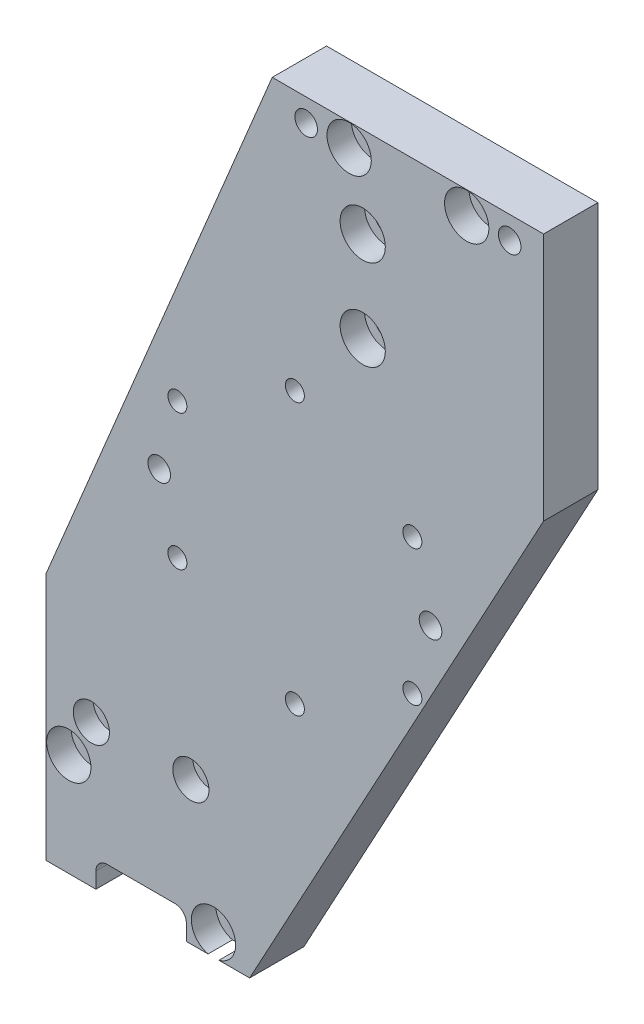
from build123d import *

# Parameters (mm, degrees)
SKETCH_1_W                   = 110
SKETCH_1_H                   = 175
EXTRUDE_1_DEPTH              = 6
CHAMFER_1_SIZE               = 50
CHAMFER_1_SIZE2              = 120
CHAMFER_2_SIZE               = 65
CHAMFER_2_SIZE2              = 120
HOLE_WIZARD_M5_1_D           = 5
HOLE_WIZARD_M5_1_2_D         = 4.2
F_5_0MM_1_D                  = 5
HOLE_WIZARD_M5_3_D           = 5.5
HOLE_WIZARD_M5_3_CBORE_D     = 9.8
HOLE_WIZARD_M5_3_CBORE_DEPTH = 5.4
HOLE_WIZARD_M5_4_D           = 5.5
HOLE_WIZARD_M5_4_CBORE_D     = 10
HOLE_WIZARD_M5_4_CBORE_DEPTH = 5.4
HOLE_WIZARD_M4_1_D           = 4.5
HOLE_WIZARD_M4_1_CBORE_D     = 8
HOLE_WIZARD_M4_1_CBORE_DEPTH = 4.4
HOLE_WIZARD_M5_6_D           = 5.5
HOLE_WIZARD_M5_6_CBORE_D     = 9.8
HOLE_WIZARD_M5_6_CBORE_DEPTH = 5.4
SKETCH_16_W                  = 20
SKETCH_16_H                  = 12
CUT_EXTRUDE_1_DEPTH          = 105.04446165
FILLET_1_R                   = 2.5


with BuildPart() as part:
    # 草图1 → 凸台-拉伸1 (new, symmetric)
    with BuildSketch(Plane.XY):
        Rectangle(SKETCH_1_W, SKETCH_1_H)
    extrude(amount=EXTRUDE_1_DEPTH, both=True)

    # 倒角1
    chamfer_1_edges = [part.edges().sort_by_distance(p)[0] for p in [
        (-55, 87.5, 0),
    ]]
    chamfer_1_side = [part.faces().sort_by_distance(p)[0] for p in [
        (0, 87.5, 0),
    ]]
    chamfer(chamfer_1_edges, length=CHAMFER_1_SIZE, length2=CHAMFER_1_SIZE2, reference=chamfer_1_side[0])

    # 倒角2
    chamfer_2_edges = [part.edges().sort_by_distance(p)[0] for p in [
        (55, -87.5, 0),
    ]]
    chamfer_2_side = [part.faces().sort_by_distance(p)[0] for p in [
        (0, -87.5, 0),
    ]]
    chamfer(chamfer_2_edges, length=CHAMFER_2_SIZE, length2=CHAMFER_2_SIZE2, reference=chamfer_2_side[0])

    # Hole Wizard M5 _1 (through all)
    with Locations(Plane.XY.offset(6)):
        with Locations((47.5, 82.5), (2.5, 82.5)):
            Hole(HOLE_WIZARD_M5_1_D / 2)

    # Hole Wizard M5 _1 2 (through all)
    with Locations(Plane.XY.offset(6)):
        with Locations((0, 30), (25.980762114, 15), (25.980762114, -15), (0, -30), (-25.980762114, -15), (-25.980762114, 15)):
            Hole(HOLE_WIZARD_M5_1_2_D / 2)

    # Ø5.0mm 暗销孔1 (through all)
    with Locations(Plane.XY.offset(6)):
        with Locations((30, 0), (-30, 0)):
            Hole(F_5_0MM_1_D / 2)

    # M5 六角凹头螺钉的柱形沉头孔3 (through all)
    with Locations(Plane.XY.offset(6)):
        with Locations((38, 82.5), (12, 82.5)):
            CounterBoreHole(HOLE_WIZARD_M5_3_D / 2, HOLE_WIZARD_M5_3_CBORE_D / 2, HOLE_WIZARD_M5_3_CBORE_DEPTH)

    # M5 六角凹头螺钉的柱形沉头孔4 (through all)
    with Locations(Plane.XY.offset(6)):
        with Locations((15, 67.5), (15, 47.5)):
            CounterBoreHole(HOLE_WIZARD_M5_4_D / 2, HOLE_WIZARD_M5_4_CBORE_D / 2, HOLE_WIZARD_M5_4_CBORE_DEPTH)

    # M4 六角凹头螺钉的柱形沉头孔1 (through all)
    with Locations(Plane.XY.offset(6)):
        with Locations((-45, -56), (-23, -56)):
            CounterBoreHole(HOLE_WIZARD_M4_1_D / 2, HOLE_WIZARD_M4_1_CBORE_D / 2, HOLE_WIZARD_M4_1_CBORE_DEPTH)

    # M5 六角凹头螺钉的柱形沉头孔6 (through all)
    with Locations(Plane.XY.offset(6)):
        with Locations((-50, -64.75), (-18, -82.75)):
            CounterBoreHole(HOLE_WIZARD_M5_6_D / 2, HOLE_WIZARD_M5_6_CBORE_D / 2, HOLE_WIZARD_M5_6_CBORE_DEPTH)

    # 草图16 → 切除-拉伸1 (cut, through all)
    with BuildSketch(Plane.XY.offset(6)):
        with Locations((-34, -87.5)):
            Rectangle(SKETCH_16_W, SKETCH_16_H)
    extrude(amount=-CUT_EXTRUDE_1_DEPTH, mode=Mode.SUBTRACT)

    # 圆角1
    fillet_1_edges = [part.edges().sort_by_distance(p)[0] for p in [
        (-24, -81.5, 0),
        (-44, -81.5, 0),
    ]]
    fillet(fillet_1_edges, radius=FILLET_1_R)


solid = part.part
